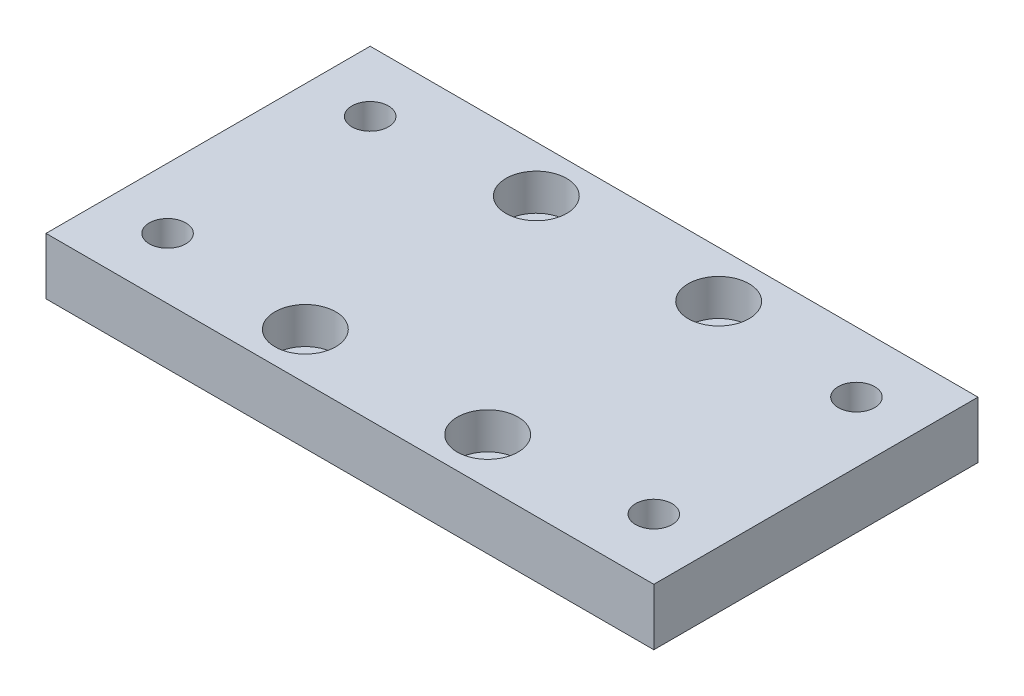
SolidWorks part; units mm, degrees
material "普通碳钢"
ref_plane "Front Plane" through (0, 0, 0) normal (0, 0, 1) x (1, 0, 0)
ref_plane "Top Plane" through (0, 0, 0) normal (0, 1, 0) x (1, 0, 0)
ref_plane "Right Plane" through (0, 0, 0) normal (1, 0, 0) x (0, 0, -1)
sketch "Sketch1" plane through (0, 0, 0) normal (0, 1, 0) x (1, 0, 0)
  line L1 (0, 0) -> (150, 0)
  line L2 (0, 0) -> (0, 80)
  line L3 (0, 80) -> (150, 80)
  line L4 (150, 0) -> (150, 80)
  dimension "D1" = 150
  dimension "D2" = 80
extrude "Boss-Extrude1" add sketch "Sketch1" along normal blind 14
hole_wizard "Hole size (% by) socket head cap screw type1" positions "Sketch2" profile "Sketch3" counterbore size "M8" standard "GB" end condition through all
sketch "Sketch2" plane through (0, 14, 0) normal (0, 1, 0) x (-1, 0, 0)
  line L0 (-52.5, -68.5) -> (-97.5, -68.5) construction
  line L1 (-97.5, -68.5) -> (-97.5, -11.5) construction
  line L2 (-97.5, -11.5) -> (-52.5, -11.5) construction
  line L3 (-52.5, -11.5) -> (-52.5, -68.5) construction
  line L5 (-75, -68.5) -> (-75, -80) construction
  line L6 (-150, -80) -> (0, -80) construction
  line L8 (-52.5, -40) -> (0, -40) construction
  line L9 (0, -80) -> (0, 0) construction
  point P0 (-52.5, -68.5)
  point P2 (-52.5, -11.5)
  point P4 (-97.5, -11.5)
  point P6 (-97.5, -68.5)
  dimension "D1" = 45
  dimension "D2" = 57
sketch "Sketch3" plane through (52.5, 14, -68.5) normal (1, 0, 0) x (0, 0, 1)
  line L0 (0, 0) -> (0, 14)
  line L1 (0, 14) -> (4.5, 14)
  line L3 (4.5, 14) -> (4.5, 9)
  line L4 (4.5, 9) -> (7.5, 9)
  line L5 (7.5, 9) -> (7.5, 0)
  line L7 (7.5, 0) -> (0, 0)
  line L11 (0, -6.35) -> (0, 107.95) construction
  dimension "通孔孔直径" = 9
  dimension "通孔孔深度" = 14
  dimension "柱形沉头孔直径" = 15
  dimension "柱形沉头孔深度" = 9
hole_wizard "Ø9.0 (9) Diameter Hole1" positions "Sketch4" profile "Sketch5" hole size "Ø9.0" standard "GB" end condition through all
sketch "Sketch4" plane through (0, 14, 0) normal (0, 1, 0) x (-1, 0, 0)
  line L0 (-15, -65) -> (-135, -65) construction
  line L1 (-135, -65) -> (-135, -15) construction
  line L2 (-135, -15) -> (-15, -15) construction
  line L3 (-15, -15) -> (-15, -65) construction
  line L5 (-75, -65) -> (-75, -80) construction
  line L6 (-150, -80) -> (0, -80) construction
  line L8 (-15, -40) -> (0, -40) construction
  line L9 (0, -80) -> (0, 0) construction
  point P0 (-15, -65)
  point P2 (-15, -15)
  point P4 (-135, -15)
  point P6 (-135, -65)
  dimension "D1" = 50
  dimension "D2" = 120
sketch "Sketch5" plane through (15, 14, -65) normal (1, 0, 0) x (0, 0, 1)
  line L0 (0, 0) -> (0, 14)
  line L1 (0, 14) -> (4.5, 14)
  line L2 (4.5, 14) -> (4.5, 0)
  line L5 (4.5, 0) -> (0, 0)
  line L11 (0, -6.35) -> (0, 107.95) construction
  dimension "通孔孔直径" = 9
  dimension "通孔孔深度" = 14
